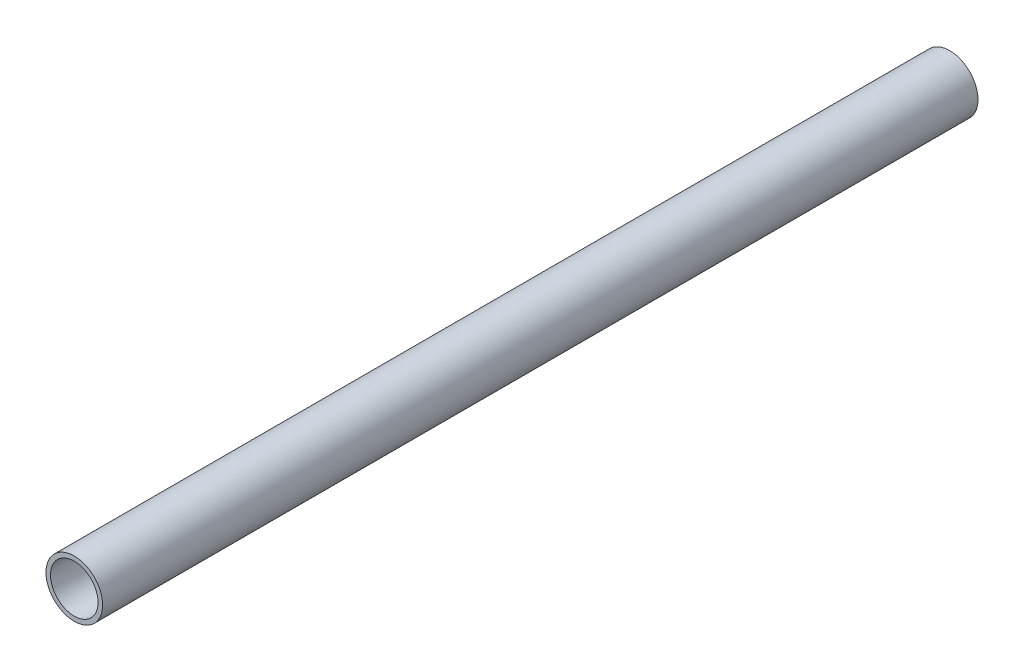
from build123d import *

# Parameters (mm, degrees)
SKETCH_1_R      = 20
EXTRUDE_1_DEPTH = 618
SHELL_1_T       = -3.2


with BuildPart() as part:
    # 草图1 → 凸台-拉伸1 (new body)
    with BuildSketch(Plane.XY):
        Circle(SKETCH_1_R)
    extrude(amount=EXTRUDE_1_DEPTH)

    # 抽壳1
    shell_1_openings = [part.faces().sort_by_distance(p)[0] for p in [
        (0, 0, 618),
        (0, 0, 0),
    ]]
    offset(amount=SHELL_1_T, openings=shell_1_openings, kind=Kind.INTERSECTION)


solid = part.part
